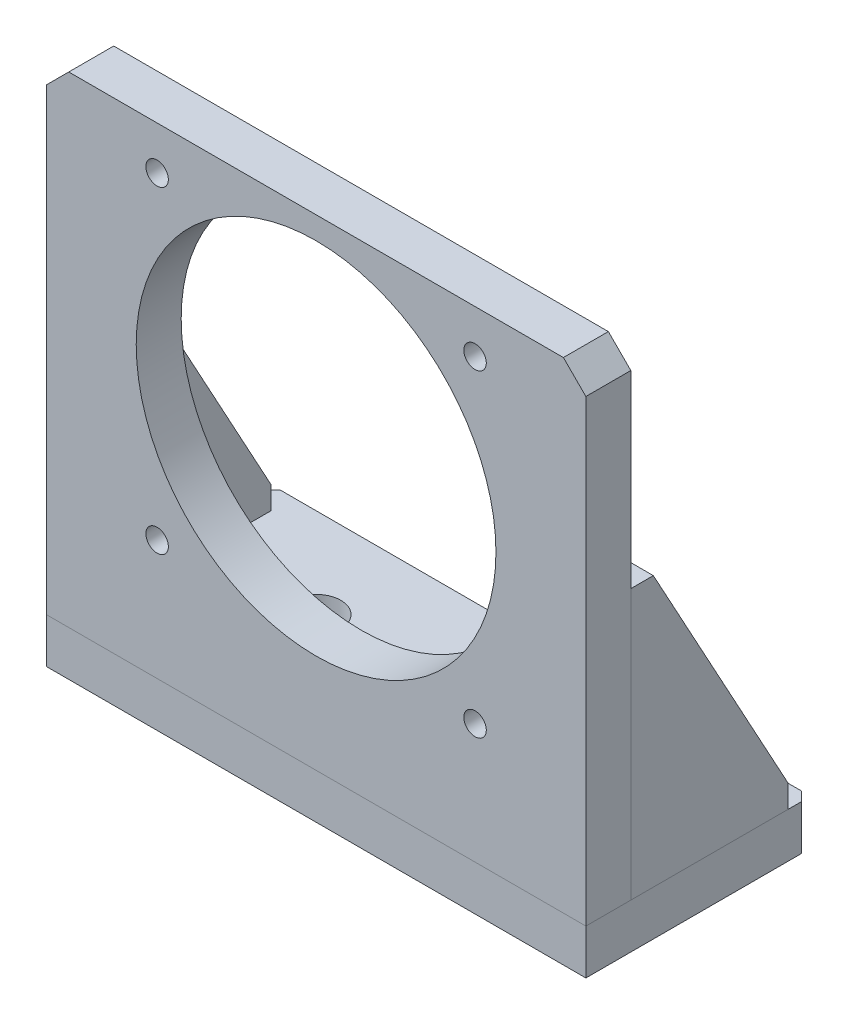
from build123d import *

# Parameters (mm, degrees)
SKETCH_1_W                   = 120
SKETCH_1_H                   = 50
EXTRUDE_1_DEPTH              = 5
SKETCH_2_W                   = 120
SKETCH_2_H                   = 10
EXTRUDE_2_DEPTH              = 107
CHAMFER_1_SIZE               = 5
CHAMFER_2_SIZE               = 2
EXTRUDE_3_DEPTH              = 5
SKETCH_4_R                   = 40
CUT_EXTRUDE_1_DEPTH          = 10
SKETCH_6_W                   = 5.5
SKETCH_6_H                   = 10
HOLE_WIZARD_M10_1_AT_2_COUNT = 2
HOLE_WIZARD_M10_1_AT_2_PITCH = 60
HOLE_WIZARD_M6_1_AT_2_COUNT  = 2
HOLE_WIZARD_M6_1_AT_2_PITCH  = 70.710678119
HOLE_WIZARD_M6_1_AT_3_COUNT  = 2
HOLE_WIZARD_M6_1_AT_3_PITCH  = 100
HOLE_WIZARD_M6_1_AT_4_COUNT  = 2
HOLE_WIZARD_M6_1_AT_4_PITCH  = 70.710678119


with BuildPart() as part:
    # 草图1 → 凸台-拉伸1 (new, symmetric)
    with BuildSketch(Plane(origin=(0, 0, 0), x_dir=(1, 0, 0), z_dir=(0, 1, 0))):
        Rectangle(SKETCH_1_W, SKETCH_1_H)
    extrude(amount=EXTRUDE_1_DEPTH, both=True)

    # 倒角2
    chamfer_2_edges = [part.edges().sort_by_distance(p)[0] for p in [
        (-60, 0, -25),
        (60, 0, -25),
    ]]
    chamfer(chamfer_2_edges, length=CHAMFER_2_SIZE)

    # 草图6 → M10 间隙孔1 (revolve, cut)
    with BuildSketch(Plane(origin=(30, 5, -5), x_dir=(0, 0, 1), z_dir=(1, 0, 0))):
        with Locations((2.75, 5)):
            Rectangle(SKETCH_6_W, SKETCH_6_H)
    hole_wizard_m10_1 = revolve(axis=Axis((30, 11.35, -5), (0, -1, 0)), mode=Mode.SUBTRACT)

    # M10 间隙孔1 at 2: M10 间隙孔1 ×2
    with Locations(*[(-i * HOLE_WIZARD_M10_1_AT_2_PITCH, 0, 0) for i in range(1, HOLE_WIZARD_M10_1_AT_2_COUNT)]):
        add(hole_wizard_m10_1, mode=Mode.SUBTRACT)


with BuildPart() as body_2:
    # 草图2 → 凸台-拉伸2 (new body)
    with BuildSketch(Plane(origin=(0, 5, 0), x_dir=(1, 0, 0), z_dir=(0, 1, 0))):
        with Locations((0, -20)):
            Rectangle(SKETCH_2_W, SKETCH_2_H)
    extrude(amount=EXTRUDE_2_DEPTH)

    # 倒角1
    chamfer_1_edges = [body_2.edges().sort_by_distance(p)[0] for p in [
        (-60, 112, 20),
        (60, 112, 20),
    ]]
    chamfer(chamfer_1_edges, length=CHAMFER_1_SIZE)

    # 草图4 → 切除-拉伸1 (cut)
    with BuildSketch(Plane.XY.offset(25)):
        with Locations((0, 67)):
            Circle(SKETCH_4_R)
    extrude(amount=-CUT_EXTRUDE_1_DEPTH, mode=Mode.SUBTRACT)

    # 草图8 → M6 螺纹孔1 (revolve, cut)
    with BuildSketch(Plane(origin=(-35.355339059, 102.355339059, 25), x_dir=(0, -1, 0), z_dir=(1, 0, 0))):
        Polygon((0, 0), (0, 16.502151548), (2.5, 15), (2.5, 0), align=None)
    hole_wizard_m6_1 = revolve(axis=Axis((-35.355339059, 102.355339059, 31.35), (0, 0, -1)), mode=Mode.SUBTRACT)

    # M6 螺纹孔1 at 2: M6 螺纹孔1 ×2
    with Locations(*[(i * HOLE_WIZARD_M6_1_AT_2_PITCH, 0, 0) for i in range(1, HOLE_WIZARD_M6_1_AT_2_COUNT)]):
        add(hole_wizard_m6_1, mode=Mode.SUBTRACT)

    # M6 螺纹孔1 at 3: M6 螺纹孔1 ×2
    with Locations(*[Vector(0.7071067811865476, -0.7071067811865476, 0) * (i * HOLE_WIZARD_M6_1_AT_3_PITCH) for i in range(1, HOLE_WIZARD_M6_1_AT_3_COUNT)]):
        add(hole_wizard_m6_1, mode=Mode.SUBTRACT)

    # M6 螺纹孔1 at 4: M6 螺纹孔1 ×2
    with Locations(*[(0, -i * HOLE_WIZARD_M6_1_AT_4_PITCH, 0) for i in range(1, HOLE_WIZARD_M6_1_AT_4_COUNT)]):
        add(hole_wizard_m6_1, mode=Mode.SUBTRACT)


with BuildPart() as body_3:
    # 草图3 → 凸台-拉伸3 (new body)
    with BuildSketch(Plane.ZY.offset(60)):
        Polygon((15, 65), (10, 65), (-20, 10), (-20, 5), (15, 5), align=None)
    extrude(amount=-EXTRUDE_3_DEPTH)


with BuildPart() as body_4:
    # 镜向1: mirrored copy
    add(body_3.part.mirror(Plane(origin=(0, 0, 0), x_dir=(0, 0, 1), z_dir=(1, 0, 0))))


solid = Compound([part.part, body_2.part, body_3.part, body_4.part])
